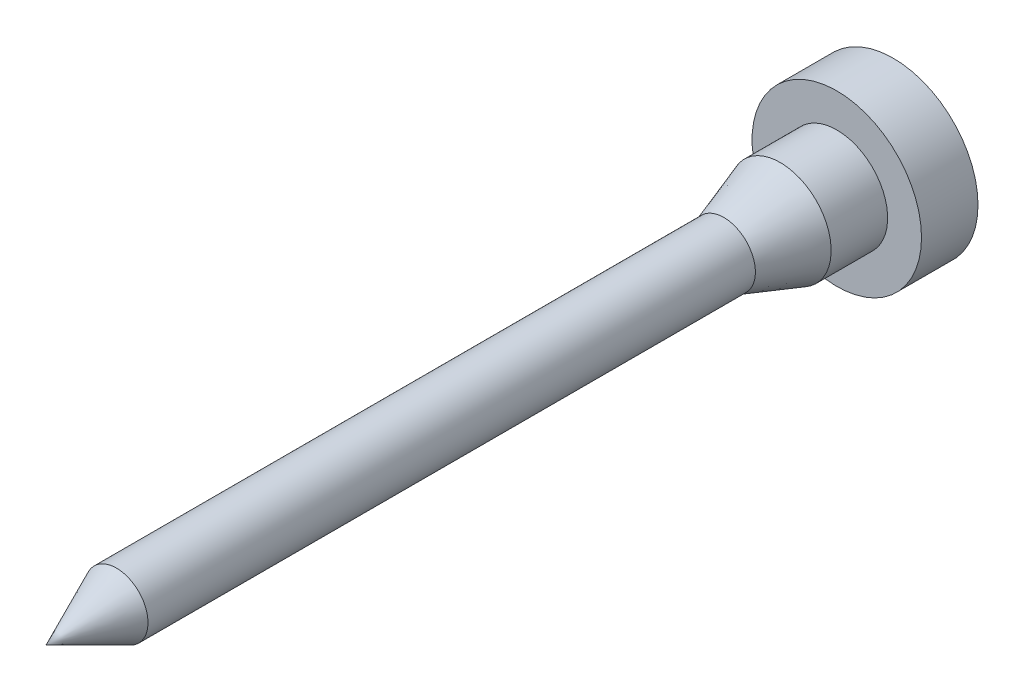
from build123d import *

# Parameters (mm, degrees)
SKETCH1_R           = 15
BOSS_EXTRUDE1_DEPTH = 10


with BuildPart() as part:
    # Sketch1 → Boss-Extrude1 (new body)
    with BuildSketch(Plane.XY):
        Circle(SKETCH1_R)
    extrude(amount=BOSS_EXTRUDE1_DEPTH)

    # Sketch2 → Revolve1 (revolve)
    with BuildSketch(Plane(origin=(0, 0, 0), x_dir=(1, 0, 0), z_dir=(0, 1, 0)), mode=Mode.PRIVATE) as revolve1_sk:
        Polygon((9, -10), (9, -20), (5.585921345, -30), (5.585921345, -137.526835229), (0, -150), (0, -10), align=None)
    revolve(revolve1_sk.sketch.rotate(Axis((0, 0, -14.229599779), (0, 0, 1)), 180), axis=Axis((0, 0, -14.229599779), (0, 0, 1)))


solid = part.part
